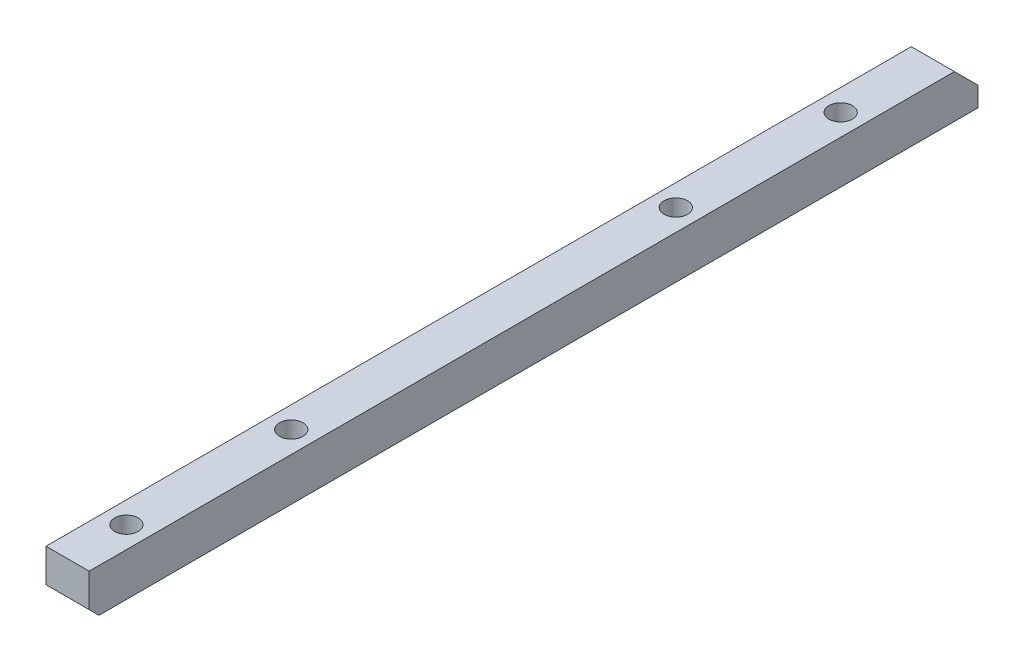
from build123d import *

# Parameters (mm, degrees)
SKETCH1_W           = 22
SKETCH1_H           = 22
BOSS_EXTRUDE1_DEPTH = 226.5
SKETCH2_R           = 6
CUT_EXTRUDE1_DEPTH  = 228.831626426
CHAMFER1_SIZE       = 5
CHAMFER2_SIZE       = 12


with BuildPart() as part:
    # Sketch1 → Boss-Extrude1 (new, symmetric)
    with BuildSketch(Plane.XY):
        Rectangle(SKETCH1_W, SKETCH1_H)
    extrude(amount=BOSS_EXTRUDE1_DEPTH, both=True)

    # Sketch2 → Cut-Extrude1 (cut, through all)
    with BuildSketch(Plane(origin=(0, 11, 0), x_dir=(1, 0, 0), z_dir=(0, 1, 0))):
        with Locations(Location((0, -196.5, 0), (0, 0, 270))):
            Circle(SKETCH2_R)
        with Locations(Location((0, -112.5, 0), (0, 0, 270))):
            Circle(SKETCH2_R)
        with Locations(Location((0, 83.5, 0), (0, 0, 270))):
            Circle(SKETCH2_R)
        with Locations(Location((0, 167.5, 0), (0, 0, 270))):
            Circle(SKETCH2_R)
    extrude(amount=-CUT_EXTRUDE1_DEPTH, mode=Mode.SUBTRACT)

    # Chamfer1
    chamfer1_edges = [part.edges().sort_by_distance(p)[0] for p in [
        (0, -11, 226.5),
    ]]
    chamfer(chamfer1_edges, length=CHAMFER1_SIZE)

    # Chamfer2
    chamfer2_edges = [part.edges().sort_by_distance(p)[0] for p in [
        (0, 11, -226.5),
    ]]
    chamfer(chamfer2_edges, length=CHAMFER2_SIZE)


solid = part.part
